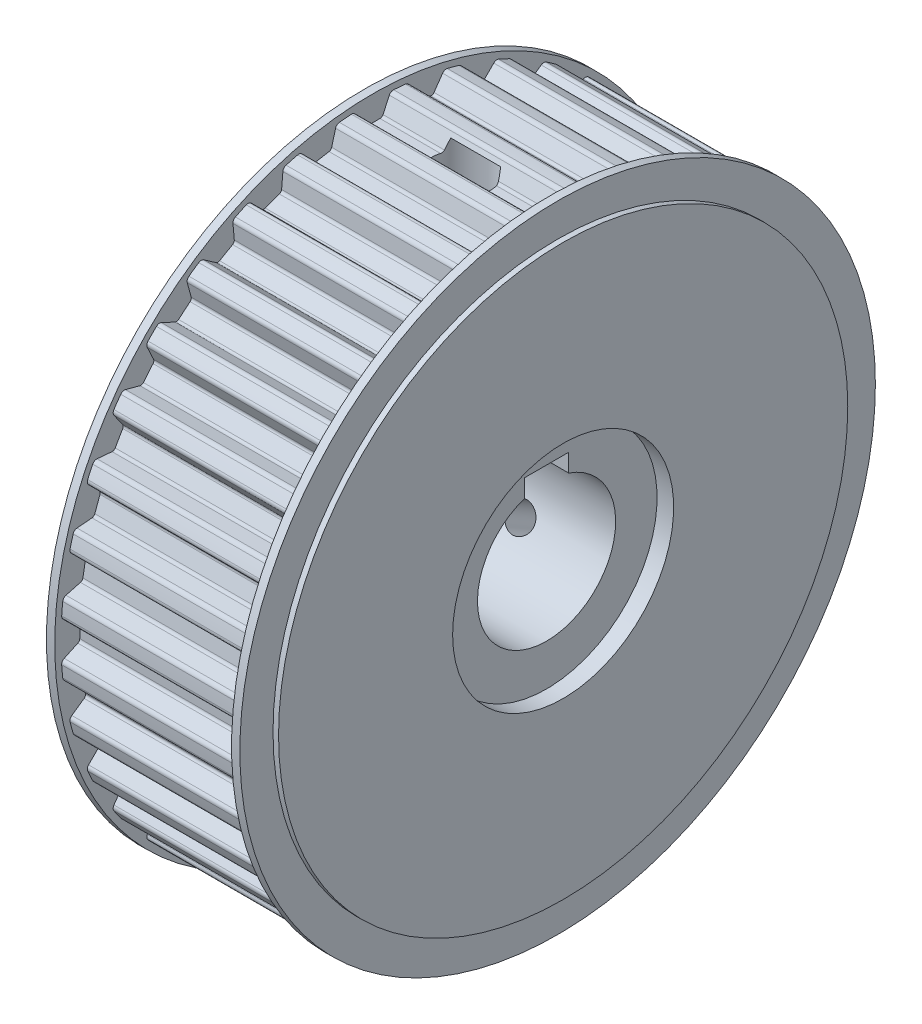
SolidWorks part; units mm, degrees
material "6061 合金"
ref_plane "前视" through (0, 0, 0) normal (0, 0, 1) x (1, 0, 0)
ref_plane "上视" through (0, 0, 0) normal (0, 1, 0) x (1, 0, 0)
ref_plane "右视" through (0, 0, 0) normal (1, 0, 0) x (0, 0, -1)
sketch "草图1" plane through (0, 0, 0) normal (1, 0, 0) x (0, 0, -1)
  line L0 (0, 56.37) -> (0, 56.751) construction
  circle A1 centre (0, 0) radius 56.37
  circle A2 centre (0, 0) radius 56.751 construction
  dimension "D2" = 112.74
  dimension "D3" = 0.381
extrude "拉伸1" add sketch "草图1" along normal mid plane 32
sketch "草图2" plane through (16, 0, 0) normal (1, 0, 0) x (0, 0, -1)
  line L0 (0, 0) -> (0, 61.5267) construction
  line L1 (-3.285, 56.2742) -> (-1.7442, 52.97)
  line L2 (-1.7442, 52.97) -> (1.7442, 52.97)
  line L3 (1.7442, 52.97) -> (3.285, 56.2742)
  circle A0 centre (0, 0) radius 56.37 construction
  arc A1 (3.285, 56.2742) -> (-3.285, 56.2742) centre (0, 0) ccw
  dimension "D2" = 3.4
  dimension "D3" = 25
  dimension "D1" = 6.57
extrude "拉伸2" cut sketch "草图2" against normal up to surface (32 mm away) up to face at (-16, 0, -56.37)
fillet "圆角1" radius 0.6 2 edges at (0, 52.97, -1.7442) (0, 52.97, 1.7442)
fillet "圆角2" radius 0.8 2 edges at (0, 56.2742, -3.285) (0, 56.2742, 3.285)
pattern_circular "阵列(圆周)1" count 36 over 360 about axis through (0, 0, 0) along (1, 0, 0) of "拉伸2", "圆角1", "圆角2"
sketch "草图6" plane through (16, 0, 0) normal (1, 0, 0) x (0, 0, -1)
  circle A0 centre (0, 0) radius 57.5
  dimension "D1" = 115
extrude "凸台-拉伸2" add sketch "草图6" along normal blind 1.5
sketch "草图7" plane through (17.5, 0, 0) normal (1, 0, 0) x (0, 0, -1)
  circle A0 centre (0, 0) radius 51.5
  dimension "D1" = 103
extrude "凸台-拉伸3" add sketch "草图7" along normal blind 1
mirror "镜向2" about plane through (0, 0, 0) normal (1, 0, 0) of "凸台-拉伸3", "凸台-拉伸2"
sketch "草图8" plane through (-18.5, 0, 0) normal (-1, 0, 0) x (0, 0, 1)
  circle A0 centre (0, 0) radius 12.5
  dimension "D1" = 25
extrude "切除-拉伸1" cut sketch "草图8" against normal through all
sketch "草图9" plane through (-18.5, 0, 0) normal (-1, 0, 0) x (0, 0, 1)
  circle A0 centre (0, 0) radius 23.5
  dimension "D1" = 47
extrude "切除-拉伸2" [suppressed] cut sketch "草图9" against normal blind 32.5
sketch "草图10" [suppressed] plane through (0, 0, 0) normal (0, 1, 0) x (1, 0, 0)
  line L0 (14, 23.5) -> (-18.5, 23.5) construction
  line L1 (-15.8, 23.5) -> (-14, 23.5)
  line L2 (-15.8, 23.5) -> (-15.8, 24.5)
  line L3 (-15.8, 24.5) -> (-14, 24.5)
  line L4 (-14, 23.5) -> (-14, 24.5)
  line L5 (14, 23.5) -> (14, -23.5) construction
  line L6 (0, 0) -> (-33.3455, 0) construction
  dimension "D1" = 1.8
  dimension "D2" = 28
  dimension "D3" = 24.5
revolve "切除-旋转1" [suppressed] cut sketch "草图10" angle 360 about L6
sketch "草图11" plane through (-18.5, 0, 0) normal (-1, 0, 0) x (0, 0, 1)
  circle A0 centre (0, 0) radius 20
  dimension "D1" = 40
extrude "切除-拉伸3" cut sketch "草图11" against normal blind 3
mirror "镜向3" about plane through (0, 0, 0) normal (1, 0, 0) of "切除-拉伸3"
sketch "草图12" plane through (-18.5, 0, 0) normal (-1, 0, 0) x (0, 0, 1)
  line L0 (0, 0) -> (0, 17.6786) construction
  line L1 (-4, 15.1) -> (4, 15.1)
  line L2 (-4, 15.1) -> (-4, 5.4071)
  line L3 (-4, 5.4071) -> (4, 5.4071)
  line L4 (4, 15.1) -> (4, 5.4071)
  line L5 (0, 0) -> (24.8621, 0) construction
  dimension "D1" = 8
  dimension "D2" = 15.1
extrude "切除-拉伸4" cut sketch "草图12" against normal through all
ref_plane "基准面1" through (0, 55, 0) normal (0, 1, 0) x (1, 0, 0)
hole_wizard "M6 螺纹孔1" positions "草图14" profile "草图13" tap size "M6" standard "GB"
sketch "草图14" plane through (0, 55, 0) normal (0, 1, 0) x (1, 0, 0)
  point P0 (0, 0)
cosmetic thread "孔螺蚊线1" parameters "D1"=12, "D2"=6
sketch "草图13" plane through (0, 55, 0) normal (1, 0, 0) x (0, 0, 1)
  line L0 (0, 0) -> (0, 51.5022)
  line L1 (0, 51.5022) -> (2.5, 50)
  line L2 (2.5, 50) -> (2.5, 0)
  line L5 (2.5, 0) -> (0, 0)
  line L10 (0, 51.5022) -> (-2.5, 50) construction
  line L11 (0, -6.35) -> (0, 107.95) construction
  dimension "螺纹孔钻头直径" = 5
  dimension "螺纹孔钻头深度" = 50
  dimension "导头角度" = 118
sketch "草图15" plane through (0, 55, 0) normal (0, 1, 0) x (1, 0, 0)
  circle A0 centre (0, 0) radius 5.25
  dimension "D1" = 10.5
extrude "切除-拉伸5" cut sketch "草图15" against normal blind 22.76
pattern_circular "阵列(圆周)2" count 2 every 120 about axis through (18.5, 0, 0) along (-1, 0, 0) of "切除-拉伸5", "M6 螺纹孔1"
